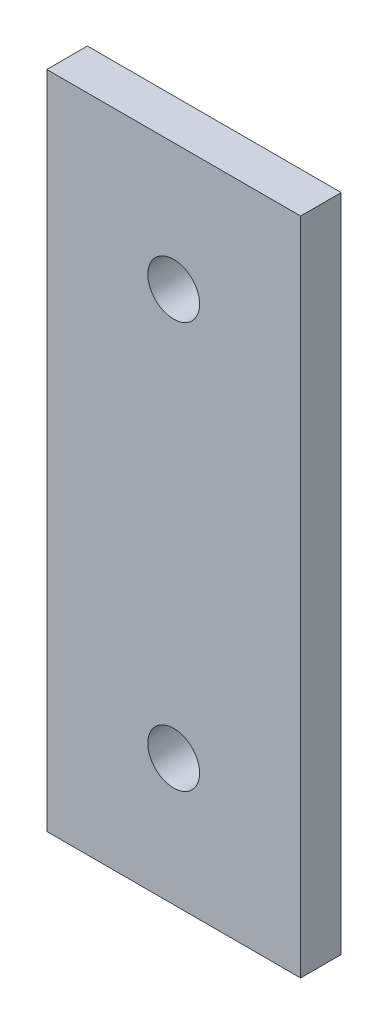
SolidWorks part; units mm, degrees
material "1023 碳钢板 (SS)"
ref_plane "Front Plane" through (0, 0, 0) normal (0, 0, 1) x (1, 0, 0)
ref_plane "Top Plane" through (0, 0, 0) normal (0, 1, 0) x (1, 0, 0)
ref_plane "Right Plane" through (0, 0, 0) normal (1, 0, 0) x (0, 0, -1)
sketch "Sketch1" plane through (0, 0, 0) normal (0, 0, 1) x (1, 0, 0)
  line L1 (-25, 65) -> (25, 65)
  line L2 (-25, 65) -> (-25, -65)
  line L3 (-25, -65) -> (25, -65)
  line L4 (25, 65) -> (25, -65)
  line L5 (-25, 65) -> (25, -65) construction
  line L6 (-25, -65) -> (25, 65) construction
  point P0 (0, 0)
  dimension "D1" = 50
  dimension "D2" = 130
extrude "Boss-Extrude1" add sketch "Sketch1" along normal blind 8
sketch "Sketch2" plane through (0, 0, 8) normal (0, 0, 1) x (1, 0, 0)
  circle A0 centre (0, 40) radius 5.097
  circle A1 centre (0, -40) radius 6.4027
  dimension "D1" = 80
  dimension "D2" = 40
hole_wizard "M12 Tapped Hole1" positions "Sketch3" profile "Sketch4" tap size "M12" standard "ISO"
sketch "Sketch3" plane through (0, 0, 8) normal (0, 0, 1) x (1, 0, 0)
  point P0 (0, 40)
  point P3 (0, -40)
sketch "Sketch4" plane through (0, 40, 8) normal (1, 0, 0) x (0, -1, 0)
  line L0 (0, 0) -> (0, 32.3144)
  line L1 (0, 32.3144) -> (5.1, 29.25)
  line L2 (5.1, 29.25) -> (5.1, 0)
  line L5 (5.1, 0) -> (0, 0)
  line L10 (0, 32.3144) -> (-5.1, 29.25) construction
  line L11 (0, -6.35) -> (0, 107.95) construction
  dimension "螺纹孔钻头直径" = 10.2
  dimension "螺纹孔钻头深度" = 29.25
  dimension "导头角度" = 118
cosmetic thread "Hole Thread Line1"
cosmetic thread "Hole Thread Line2"
